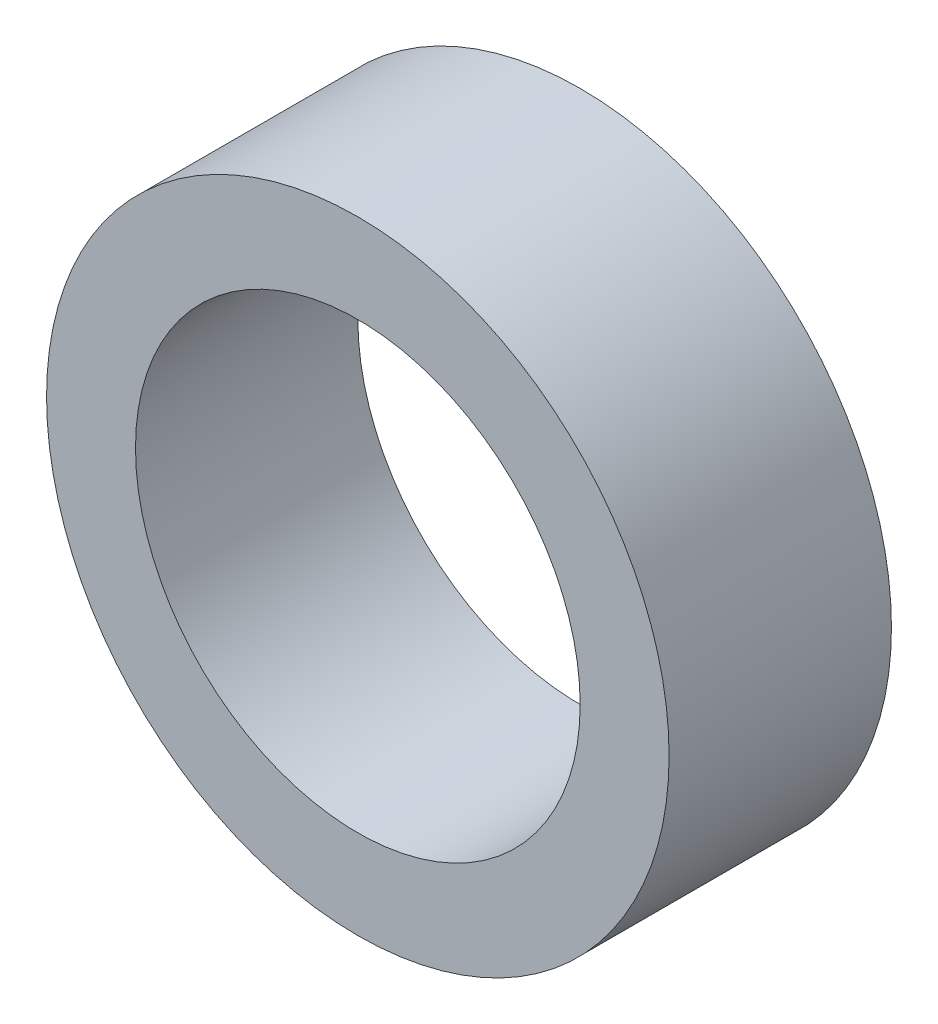
from build123d import *

# Parameters (mm, degrees)
SKETCH_2_R      = 14
SKETCH_2_R_2    = 10
EXTRUDE_1_DEPTH = 10


with BuildPart() as part:
    # 草图2 → 凸台-拉伸1 (new body)
    with BuildSketch(Plane.XY):
        Circle(SKETCH_2_R)
        Circle(SKETCH_2_R_2, mode=Mode.SUBTRACT)
    extrude(amount=EXTRUDE_1_DEPTH)


solid = part.part
